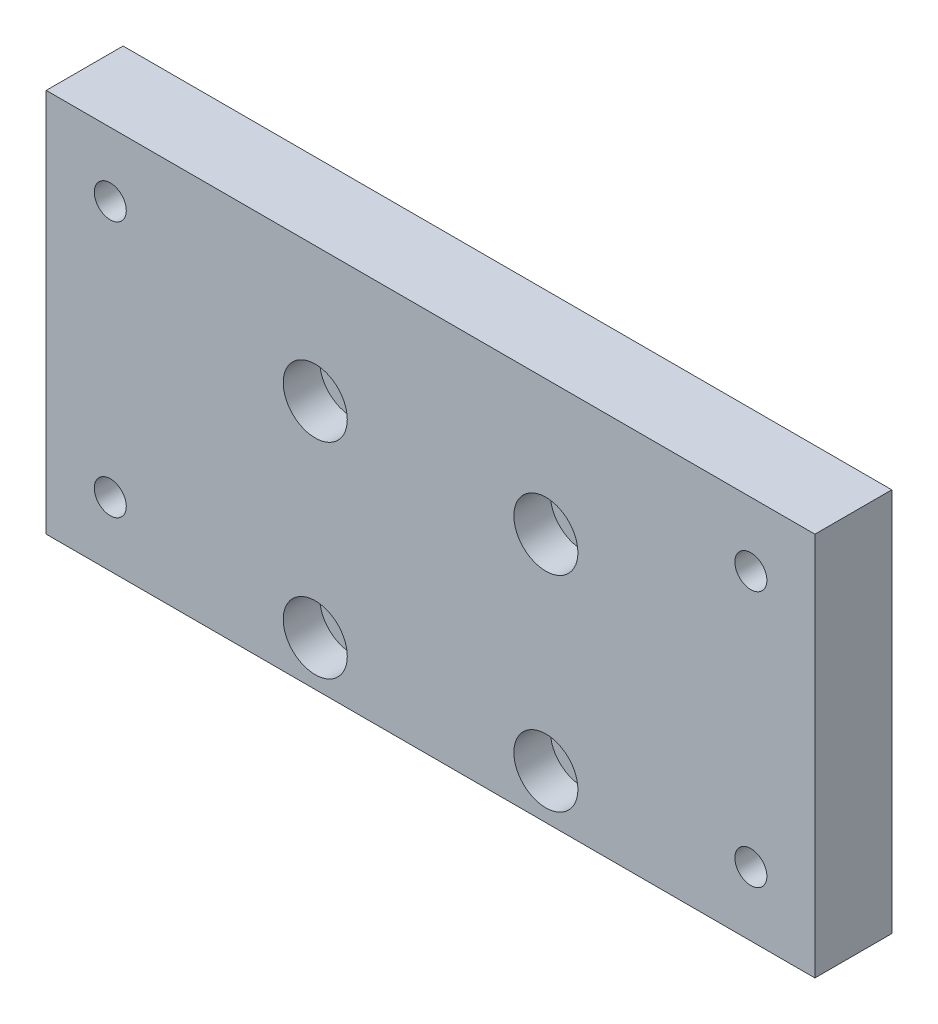
from build123d import *

# Parameters (mm, degrees)
SKETCH1_W                                         = 120
SKETCH1_H                                         = 60
SKETCH1_R                                         = 1.5
BOSS_EXTRUDE1_DEPTH                               = 12
HOLE_SIZE_PER_HEX_SOCKET_SCREW_TYPE_1_D           = 5.5
HOLE_SIZE_PER_HEX_SOCKET_SCREW_TYPE_1_DEPTH       = 18
HOLE_SIZE_PER_HEX_SOCKET_SCREW_TYPE_1_CBORE_D     = 10
HOLE_SIZE_PER_HEX_SOCKET_SCREW_TYPE_1_CBORE_DEPTH = 5.7
HOLE_SIZE_PER_HEX_SOCKET_SCREW_TYPE_1_TIP         = 1.652366702
M6_TAPPED_HOLE1_D                                 = 5
M6_TAPPED_HOLE1_DEPTH                             = 15
M6_TAPPED_HOLE1_TIP                               = 1.502151548


with BuildPart() as part:
    # Sketch1 → Boss-Extrude1 (new body)
    with BuildSketch(Plane.XY):
        Rectangle(SKETCH1_W, SKETCH1_H)
        with Locations((-50, 20)):
            Circle(SKETCH1_R, mode=Mode.SUBTRACT)
        with Locations((50, 20)):
            Circle(SKETCH1_R, mode=Mode.SUBTRACT)
        with Locations((50, -20)):
            Circle(SKETCH1_R, mode=Mode.SUBTRACT)
        with Locations((-50, -20)):
            Circle(SKETCH1_R, mode=Mode.SUBTRACT)
    extrude(amount=BOSS_EXTRUDE1_DEPTH)

    # Hole Size (per hex socket screw type)1
    with Locations(Plane(origin=(-18, 9, 12), x_dir=(1, 0, 0), z_dir=(0, 0, 1))):
        with Locations((0, 0), (36, 0), (0, -32), (36, -32)):
            CounterBoreHole(HOLE_SIZE_PER_HEX_SOCKET_SCREW_TYPE_1_D / 2, HOLE_SIZE_PER_HEX_SOCKET_SCREW_TYPE_1_CBORE_D / 2, HOLE_SIZE_PER_HEX_SOCKET_SCREW_TYPE_1_CBORE_DEPTH, depth=HOLE_SIZE_PER_HEX_SOCKET_SCREW_TYPE_1_DEPTH)
            with Locations((0, 0, -(HOLE_SIZE_PER_HEX_SOCKET_SCREW_TYPE_1_DEPTH + HOLE_SIZE_PER_HEX_SOCKET_SCREW_TYPE_1_TIP / 2))):  # 118° drill point
                Cone(0, HOLE_SIZE_PER_HEX_SOCKET_SCREW_TYPE_1_D / 2, HOLE_SIZE_PER_HEX_SOCKET_SCREW_TYPE_1_TIP, mode=Mode.SUBTRACT)

    # M6 Tapped Hole1
    with Locations(Plane.XY.offset(12)):
        with Locations((-50, 20), (-50, -20), (50, -20), (50, 20)):
            Hole(M6_TAPPED_HOLE1_D / 2, depth=M6_TAPPED_HOLE1_DEPTH)
            with Locations((0, 0, -(M6_TAPPED_HOLE1_DEPTH + M6_TAPPED_HOLE1_TIP / 2))):  # 118° drill point
                Cone(0, M6_TAPPED_HOLE1_D / 2, M6_TAPPED_HOLE1_TIP, mode=Mode.SUBTRACT)


solid = part.part
